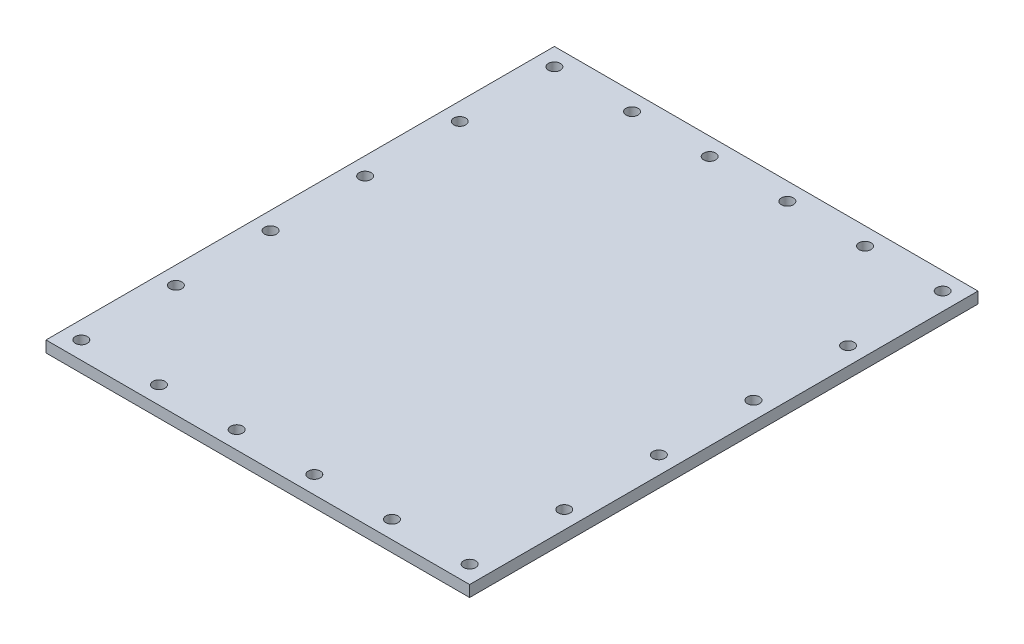
SolidWorks part; units mm, degrees
material "Q235B"
ref_plane "Front Plane" through (0, 0, 0) normal (0, 0, 1) x (1, 0, 0)
ref_plane "Top Plane" through (0, 0, 0) normal (0, 1, 0) x (1, 0, 0)
ref_plane "Right Plane" through (0, 0, 0) normal (1, 0, 0) x (0, 0, -1)
sketch "Sketch1" plane through (0, 0, 0) normal (0, 1, 0) x (1, 0, 0)
  line L1 (300, -360) -> (-300, -360)
  line L2 (300, -360) -> (300, 360)
  line L3 (300, 360) -> (-300, 360)
  line L4 (-300, -360) -> (-300, 360)
  line L5 (300, -360) -> (-300, 360) construction
  line L6 (300, 360) -> (-300, -360) construction
  point P0 (0, 0)
  dimension "D1" = 720
  dimension "D2" = 600
extrude "Boss-Extrude1" add sketch "Sketch1" along normal mid plane 16
hole_wizard "Ø17.0 (17) Diameter Hole1" positions "Sketch2" profile "Sketch3" hole size "Ø17.0" standard "GB" end condition up to next
sketch "Sketch2" plane through (0, 8, 0) normal (0, 1, 0) x (1, 0, 0)
  line L0 (-275, -335) -> (-165, -335) construction
  line L1 (0, 360) -> (0, 0) construction
  line L2 (300, 360) -> (-300, 360) construction
  line L3 (0, 0) -> (300, 0) construction
  line L4 (300, -360) -> (300, 360) construction
  point P0 (-275, -335)
  point P5 (-165, -335)
  point P6 (-55, -335)
  point P7 (55, -335)
  point P8 (165, -335)
  point P9 (275, -335)
  point P16 (-275, -201)
  point P17 (-275, -67)
  point P18 (-275, 67)
  point P19 (-275, 201)
  point P20 (-275, 335)
  point P30 (275, 335)
  point P31 (165, 335)
  point P32 (55, 335)
  point P33 (-55, 335)
  point P34 (-165, 335)
  point P35 (275, 201)
  point P36 (275, 67)
  point P37 (275, -67)
  point P38 (275, -201)
  dimension "D2" = 110
  dimension "D4" = 134
  dimension "D1" = 6
  dimension "D3" = 6
sketch "Sketch3" plane through (-275, 8, 335) normal (1, 0, 0) x (0, 0, 1)
  line L0 (0, 0) -> (0, 16)
  line L1 (0, 16) -> (8.5, 16)
  line L2 (8.5, 16) -> (8.5, 0)
  line L5 (8.5, 0) -> (0, 0)
  line L11 (0, -6.35) -> (0, 107.95) construction
  dimension "通孔孔直径" = 17
  dimension "通孔孔深度" = 16
